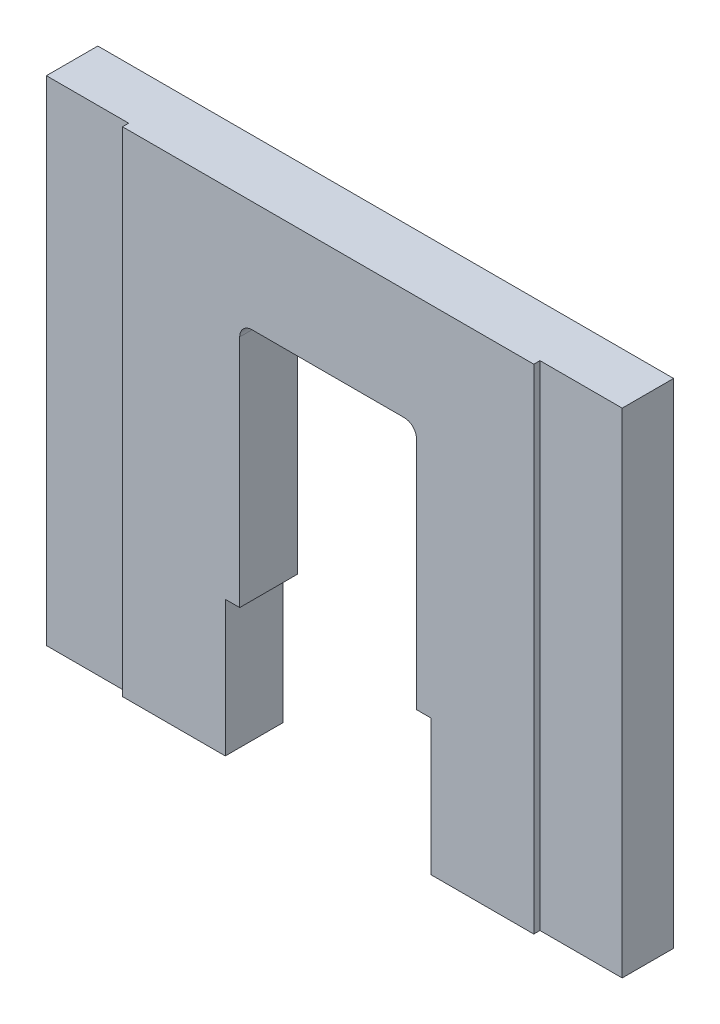
from build123d import *

# Parameters (mm, degrees)
SKETCH_1_W                      = 140
SKETCH_1_H                      = 120
EXTRUDE_1_DEPTH                 = 14
SKETCH_2_W                      = 20
SKETCH_2_H                      = 120
CUT_EXTRUDE_1_DEPTH             = 1.5
CUT_EXTRUDE_2_REACH             = 95.252
SKETCH_3_W                      = 50
SKETCH_3_H                      = 33
CUT_EXTRUDE_3_REACH             = 95.252
SKETCH_4_W                      = 43
SKETCH_4_H                      = 60
CUT_EXTRUDE_3_DIRECTION_2_DEPTH = 94.252345815
FILLET_1_R                      = 3


with BuildPart() as part:
    # 草图1 → 凸台-拉伸1 (new body)
    with BuildSketch(Plane.XY):
        Rectangle(SKETCH_1_W, SKETCH_1_H)
    extrude(amount=EXTRUDE_1_DEPTH)

    # 草图2 → 切除-拉伸1 (cut)
    with BuildSketch(Plane.XY.offset(14)):
        with Locations((-60, 0)):
            Rectangle(SKETCH_2_W, SKETCH_2_H)
        with Locations((60, 0)):
            Rectangle(SKETCH_2_W, SKETCH_2_H)
    extrude(amount=-CUT_EXTRUDE_1_DEPTH, mode=Mode.SUBTRACT)

    # 草图3 → 切除-拉伸2 (cut, up to next)
    with BuildSketch(Plane.XY.offset(14), mode=Mode.PRIVATE) as cut_extrude_2_sk1:
        with Locations((0, -43.5)):
            Rectangle(SKETCH_3_W, SKETCH_3_H)
    cut_extrude_2_tool1 = extrude(cut_extrude_2_sk1.sketch, amount=-CUT_EXTRUDE_2_REACH, mode=Mode.PRIVATE) & part.part
    add(cut_extrude_2_tool1.solids().sort_by_distance((0, -43.5, 14))[0], mode=Mode.SUBTRACT)

    # 草图4 → 切除-拉伸3 (cut, up to next)
    with BuildSketch(Plane(origin=(0, 0, 0), x_dir=(-1, 0, 0), z_dir=(0, 0, -1)), mode=Mode.PRIVATE) as cut_extrude_3_sk1:
        with Locations((0, 3)):
            Rectangle(SKETCH_4_W, SKETCH_4_H)
    cut_extrude_3_tool1 = extrude(cut_extrude_3_sk1.sketch, amount=-CUT_EXTRUDE_3_REACH, mode=Mode.PRIVATE) & part.part
    add(cut_extrude_3_tool1.solids().sort_by_distance((0, 3, 0))[0], mode=Mode.SUBTRACT)

    # 草图4 → 切除-拉伸3 direction 2 (cut)
    with BuildSketch(Plane(origin=(0, 0, 0), x_dir=(-1, 0, 0), z_dir=(0, 0, -1))):
        with Locations((0, 3)):
            Rectangle(SKETCH_4_W, SKETCH_4_H)
    extrude(amount=CUT_EXTRUDE_3_DIRECTION_2_DEPTH, mode=Mode.SUBTRACT)

    # 圆角1
    fillet_1_edges = [part.edges().sort_by_distance(p)[0] for p in [
        (-21.5, 33, 7),
        (21.5, 33, 7),
    ]]
    fillet(fillet_1_edges, radius=FILLET_1_R)


solid = part.part
